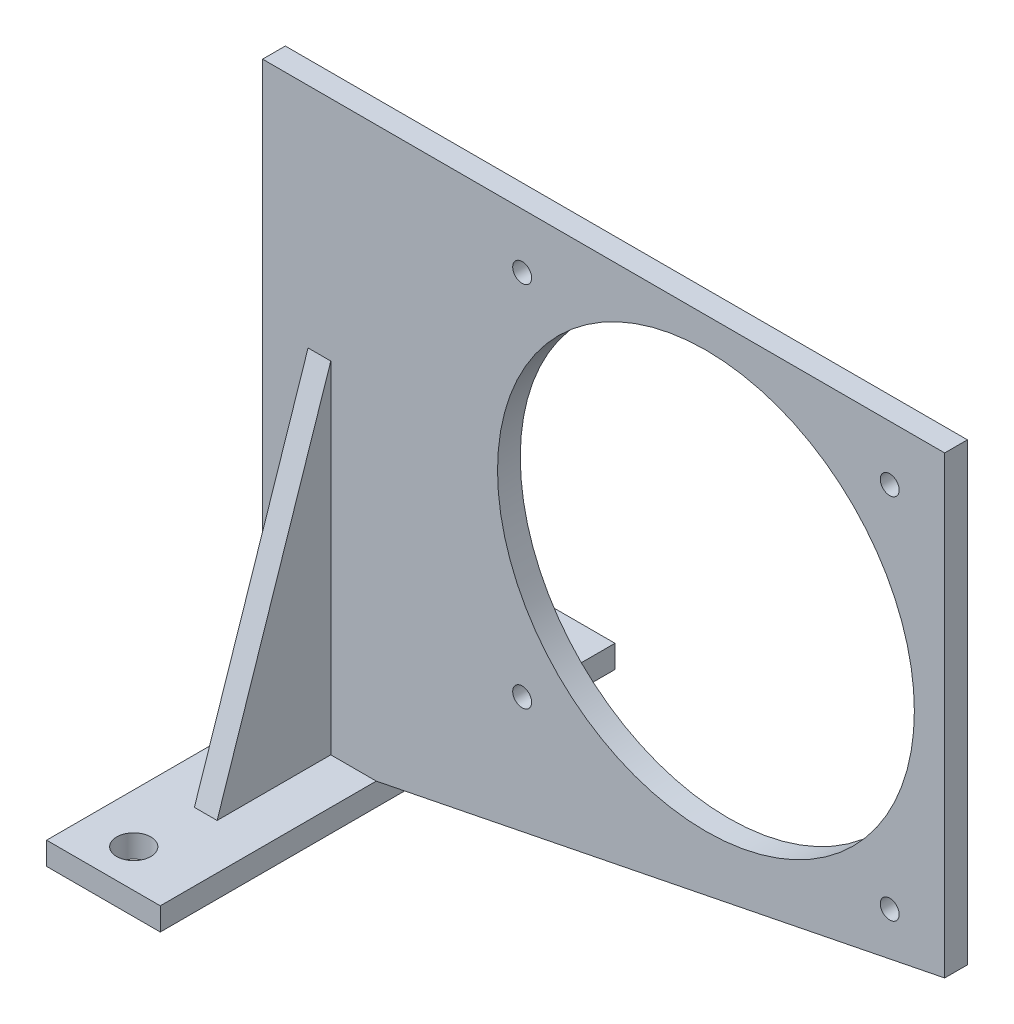
from build123d import *

# Parameters (mm, degrees)
SKETCH_1_R           = 2.5
SKETCH_1_R_2         = 55
EXTRUDE_1_DEPTH      = 6
SKETCH_4_W           = 30
SKETCH_4_H           = 120
EXTRUDE_3_DEPTH      = 6
SKETCH_5_R           = 4.5
CUT_EXTRUDE_1_DEPTH  = 6
EXTRUDE_4_DEPTH      = 3
EXTRUDE_4_DEPTH_BACK = 3


with BuildPart() as part:
    # 草图1 → 凸台-拉伸1 (new body)
    with BuildSketch(Plane.XY):
        Polygon((0, 0), (30, 0), (180, 30), (180, 150), (0, 150), align=None)
        with Locations((165.5, 135.5)):
            Circle(SKETCH_1_R, mode=Mode.SUBTRACT)
        with Locations((68.5, 135.5)):
            Circle(SKETCH_1_R, mode=Mode.SUBTRACT)
        with Locations((165.5, 38.5)):
            Circle(SKETCH_1_R, mode=Mode.SUBTRACT)
        with Locations((68.5, 38.5)):
            Circle(SKETCH_1_R, mode=Mode.SUBTRACT)
        with Locations((117, 87)):
            Circle(SKETCH_1_R_2, mode=Mode.SUBTRACT)
    extrude(amount=EXTRUDE_1_DEPTH)

    # 草图4 → 凸台-拉伸3 (add)
    with BuildSketch(Plane.XZ):
        with Locations((15, 3)):
            Rectangle(SKETCH_4_W, SKETCH_4_H)
    extrude(amount=EXTRUDE_3_DEPTH)

    # 草图5 → 切除-拉伸1 (cut)
    with BuildSketch(Plane(origin=(0, 0, 0), x_dir=(1, 0, 0), z_dir=(0, 1, 0))):
        with Locations(Location((13, 47, 0), (0, 0, 270))):
            Circle(SKETCH_5_R)
        with Locations(Location((13, -53, 0), (0, 0, 270))):
            Circle(SKETCH_5_R)
    extrude(amount=-CUT_EXTRUDE_1_DEPTH, mode=Mode.SUBTRACT)

    # 草图6 → 凸台-拉伸4 (add, two sides: drawn at the far end of the back side and taken through both)
    with BuildSketch(Plane.ZY.offset(-15).offset(-EXTRUDE_4_DEPTH_BACK)):
        Polygon((0, 90), (-30, 0), (0, 0), align=None)
        Polygon((6, 0), (6, 90), (36, 0), align=None)
    extrude(amount=EXTRUDE_4_DEPTH + EXTRUDE_4_DEPTH_BACK)


solid = part.part
